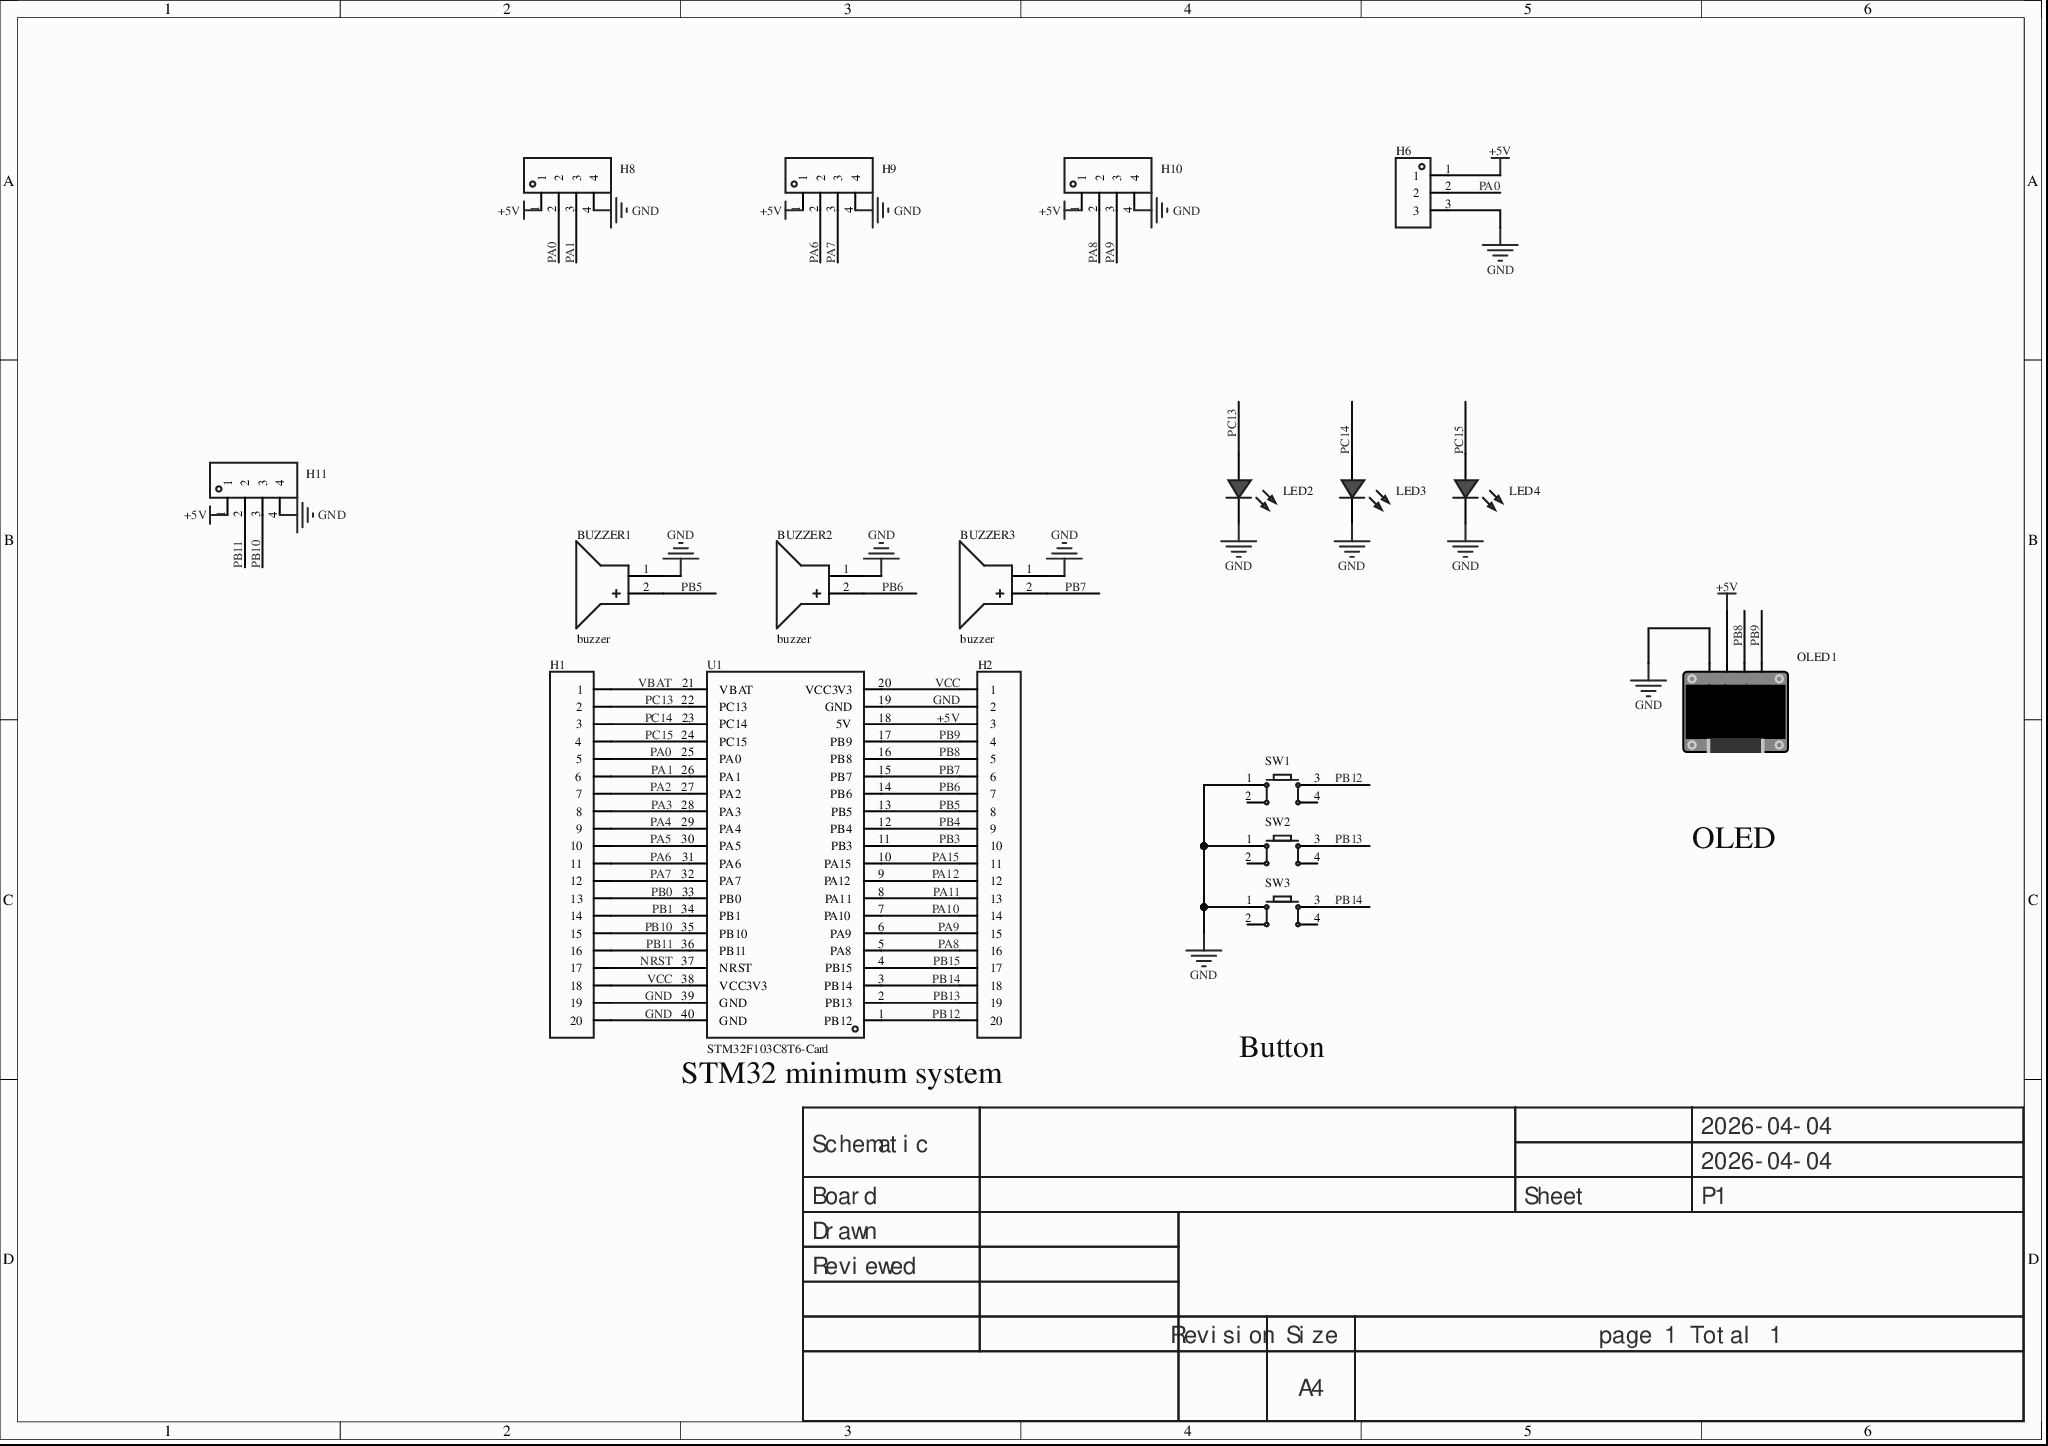
[diagram p0: MISC51974-3.schdoc]
# Altium project MISC51974-2.PrjPcb
1 sheet, 18 parts. Net scope: global (net labels, ports and power ports of the same name join across sheets).
Board file: MISC51974.pcbdoc

## Sheet MISC51974-3.schdoc
size 297 x 209 mm; Version: V1.0; @Project Name: MISC51974; @Page Count: 1; @Update Date: 2026-04-04; @Create Date: 2026-04-04; @Schematic Name: MISC51974; @Page No: 1; @Create Time: 18:58:15; @Update Time: 22:44:58; @Board Name: MISC51974

### Parts
BUZZER1  buzzer  [BUZ-TH_BD12.0-P6.00-D0.9-RD]
BUZZER2  buzzer  [BUZ-TH_BD12.0-P6.00-D0.9-RD]
BUZZER3  buzzer  [BUZ-TH_BD12.0-P6.00-D0.9-RD]
H1  (no value)  [HDR-TH_20P-P2.54-V-F]
H2  (no value)  [HDR-TH_20P-P2.54-V-F]
H6  (no value)  [HDR-TH_3P-P2.54-V-F]
H8  (no value)  [HDR-TH_4P-P2.54-V-F]
H9  (no value)  [HDR-TH_4P-P2.54-V-F]
H10  (no value)  [HDR-TH_4P-P2.54-V-F]
H11  (no value)  [HDR-TH_4P-P2.54-V-F]
LED2  (no value)  [LED-TH_5mm]
LED3  (no value)  [LED-TH_5mm]
LED4  (no value)  [LED-TH_5mm]
OLED1  (no value)  [0.96OLED_4P]
SW1  (no value)  [SW-TH_4P-L6.0-W6.0-P4.50-LS6.5]
SW2  (no value)  [SW-TH_4P-L6.0-W6.0-P4.50-LS6.5]
SW3  (no value)  [SW-TH_4P-L6.0-W6.0-P4.50-LS6.5]
U1  STM32F103C8T6-Card  [CONN-TH_L53.3-W22.9_STM32F103C8T6-CARD]

### Nets
+5V: H2.3 H6.1 H8.1 H9.1 H10.1 H11.1 OLED1.2(VCC) U1.18(5V)
GND: BUZZER1.1(-) BUZZER2.1(-) BUZZER3.1(-) H1.19 H1.20 H2.2 H6.3 H8.4 H9.4 H10.4 H11.4 LED2.2(A) LED3.2(A) LED4.2(A) OLED1.1(GND) SW1.1 SW2.1 SW3.1 U1.19(GND) U1.39(GND) U1.40(GND)
NRST: H1.17 U1.37(NRST)
PA0: H1.5 H6.2 H8.2 U1.25(PA0)
PA1: H1.6 H8.3 U1.26(PA1)
PA2: H1.7 U1.27(PA2)
PA3: H1.8 U1.28(PA3)
PA4: H1.9 U1.29(PA4)
PA5: H1.10 U1.30(PA5)
PA6: H1.11 H9.2 U1.31(PA6)
PA7: H1.12 H9.3 U1.32(PA7)
PA8: H2.16 H10.2 U1.5(PA8)
PA9: H2.15 H10.3 U1.6(PA9)
PA10: H2.14 U1.7(PA10)
PA11: H2.13 U1.8(PA11)
PA12: H2.12 U1.9(PA12)
PA15: H2.11 U1.10(PA15)
PB0: H1.13 U1.33(PB0)
PB1: H1.14 U1.34(PB1)
PB3: H2.10 U1.11(PB3)
PB4: H2.9 U1.12(PB4)
PB5: BUZZER1.2(+) H2.8 U1.13(PB5)
PB6: BUZZER2.2(+) H2.7 U1.14(PB6)
PB7: BUZZER3.2(+) H2.6 U1.15(PB7)
PB8: H2.5 OLED1.3(SCL) U1.16(PB8)
PB9: H2.4 OLED1.4(SDA) U1.17(PB9)
PB10: H1.15 H11.3 U1.35(PB10)
PB11: H1.16 H11.2 U1.36(PB11)
PB12: H2.20 SW1.3 U1.1(PB12)
PB13: H2.19 SW2.3 U1.2(PB13)
PB14: H2.18 SW3.3 U1.3(PB14)
PB15: H2.17 U1.4(PB15)
PC13: H1.2 LED2.1(C) U1.22(PC13)
PC14: H1.3 LED3.1(C) U1.23(PC14)
PC15: H1.4 LED4.1(C) U1.24(PC15)
VBAT: H1.1 U1.21(VBAT)
VCC: H1.18 H2.1 U1.20(VCC3V3) U1.38(VCC3V3)

Not connected (* = marked no-connect by the designer): SW1 2 4; SW2 2 4; SW3 2 4

### Notes on the sheet
- OLED
- STM32 minimum system
- Button
- 2026-04-04
- Schematic
- Board
- Sheet
- P1
- Drawn
- Reviewed
- Revision
- Size
- A4
- page 1 Total 1

### Library data of the parts
BUZZER1-BUZZER3 = buzzer: AddInBom: yes; ModelId: af17e4151ed84fc2a628230bf23763630819f05c4eef4c71ace90d822a990e87; ModelTransform: 472.44,472.176,0,270,0,0,0,0,-196.85; Symbol: BUZZER; Device: buzzer; LCSC Part Name: buzzer; SupplierPart: C9900014030; ManufacturerPart: buzzer; Supplier Footprint: buzzer; JLCPCB Part Class: Extended Part; Supplier: LCSC; ConvertToPcb: yes; FootprintName: BUZ-TH_BD12.0-P6.00-D0.9-RD; ModelName: BUZ-TH_BD12.0-P6.00-D0.9-RD
H1 H2 = HDR-F_2.54_1x20P: ConvertToPcb: yes; ModelId: db7015f7ad9d48b8a3b1188db02e3429; ModelName: HDR-F-2.54_1x20; ModelTransform: 1999.996,100,0,0,0,0,0,0,-118.11; Symbol: HDR-F_2.54_1x20P; Device: HDR-F_2.54_1x20P; AddInBom: yes; SupplierPart: C50984; Supplier Footprint: 插件; FootprintName: HDR-TH_20P-P2.54-V-F
H6 = HDR-F_2.54_1x3P: Symbol: PM254V-11-03-H85; 3D Model: f3b3cc5aae9641bf9e56fc160cef875b; 3D Model Transform: 299.9994,100,0,0,0,0,0,0,-118.11; ConvertToPcb: yes; ModelName: HDR2.54-F-LI-1X3P; Device: HDR-F_2.54_1x3P; Supplier Part: C541850; Supplier Footprint: 插件; AddInBom: yes; FootprintName: HDR-TH_3P-P2.54-V-F
H8-H11 = HDR-F_2.54_1x4P: Symbol: 2.54-1*4P female; 3D Model: d187812051054f85879fcaa51a310d8e0819f05c4eef4c71ace90d822a990e87; 3D Model Transform: 419.6842,98.464,0,0,0,0,0,0,-118.11; ConvertToPcb: yes; Device: HDR-F_2.54_1x4P; Supplier Part: C2718488; Supplier Footprint: 插件; AddInBom: yes; FootprintName: HDR-TH_4P-P2.54-V-F; ModelName: HDR-TH_4P-P2.54-V-F
LED2-LED4 = LED_TH-R_5mm: 3D Model: fe9cea1bdf7642cd8d9a5077ed0e2b580819f05c4eef4c71ace90d822a990e87; 3D Model Transform: 222.16,238.98,581.81,180,0,0,-6,0,-220; ConvertToPcb: yes; ModelName: LED-TH_BD5.9-P2.54-RD_RED; Symbol: LED_TH-R; Device: LED_TH-R_5mm; Supplier Footprint: 插件; AddInBom: yes; FootprintName: LED-TH_5mm
OLED1 = 0.96OLED模块_4P: Symbol: 0.96OLED module_4P; 3D Model: 79c000fdb68d45a296c2e9bedf4f9055; 3D Model Transform: 1393.69792,1318.895,0,0,0,0,0,-560.079,-137.795; ConvertToPcb: yes; Device: 0.96OLED module_4P; Supplier Footprint: 插件; AddInBom: yes; FootprintName: 0.96OLED_4P; ModelName: 0.96OLED_4P
SW1-SW3 = Key_TH_6x6x6: Contact current: 50mA; rated voltage (DC): 12V; insulation resistance: 100MΩ; circuit structure: SPST; mounting: through-hole; button shape: round button; button/cap colour: black; actuating force: 260gf@±30gf; operating temperature: -25℃~+70℃; pin style: PC pin; switch length: 6mm; switch width: 6mm; switch height: 6mm; with bracket: no;; Symbol: Tactile switch; 3D Model: 20eee248bc684ccd8cbdbb1d0d91ec6f0819f05c4eef4c71ace90d822a990e87; 3D Model Transform: 236.22,323.03,0,90,0,0,0,0,-137.795; AddInBom: yes; ModelName: SW-TH_4P-L6.0-W6.0-H5.0-LS6.5-P4.50; Device: Key_TH_6x6x6; Supplier Footprint: 插件; ConvertToPcb: yes; FootprintName: SW-TH_4P-L6.0-W6.0-P4.50-LS6.5
U1 = STM32F103C8T6-Card: AddInBom: yes; Symbol: STM32F103C8T6-CARD; Device: STM32F103C8T6-Card; LCSC Part Name: STM32F103C8T6-Card; SupplierPart: C9900077949; ManufacturerPart: STM32F103C8T6-Card; Supplier Footprint: 插件; Supplier: LCSC; ConvertToPcb: yes; FootprintName: CONN-TH_L53.3-W22.9_STM32F103C8T6-CARD